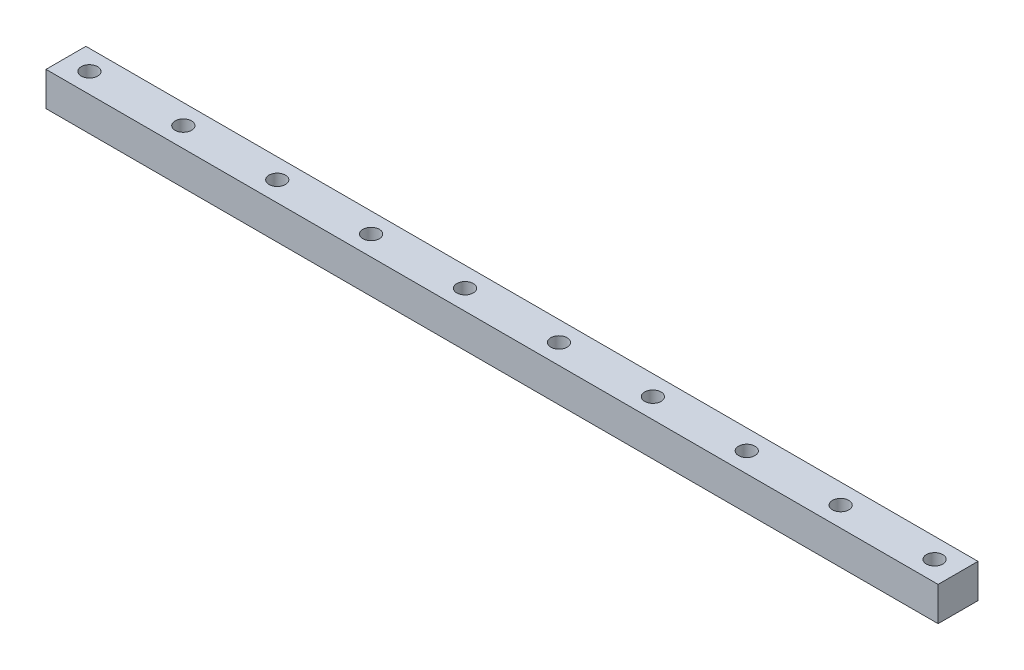
SolidWorks part; units mm, degrees
ref_plane "前视基准面" through (0, 0, 0) normal (0, 0, 1) x (1, 0, 0)
ref_plane "上视基准面" through (0, 0, 0) normal (0, 1, 0) x (1, 0, 0)
ref_plane "右视基准面" through (0, 0, 0) normal (1, 0, 0) x (0, 0, -1)
sketch "草图1" plane through (0, 0, 0) normal (0, 1, 0) x (1, 0, 0)
  line L1 (0, 0) -> (760, 0)
  line L2 (0, 0) -> (0, 34)
  line L3 (0, 34) -> (760, 34)
  line L4 (760, 0) -> (760, 34)
  dimension "D1" = 760
  dimension "D2" = 34
extrude "拉伸1" add sketch "草图1" along normal blind 29
sketch "草图2" plane through (0, 29, 0) normal (0, 1, 0) x (-1, 0, 0)
  line L0 (-760, -17) -> (0, -17) construction
  line L1 (-760, 0) -> (-760, -34) construction
  line L2 (0, -34) -> (0, 0) construction
  line L3 (-20, -34) -> (-20, 0) construction
  line L4 (-760, -34) -> (0, -34) construction
  line L5 (0, 0) -> (-760, 0) construction
  circle A0 centre (-20, -17) radius 7
  dimension "D1" = 20
extrude "切除-拉伸1" cut sketch "草图2" against normal blind 12
sketch "草图3" plane through (0, 17, 0) normal (0, 1, 0) x (-1, 0, 0)
  circle A0 centre (-20, -17) radius 4.5
extrude "切除-拉伸2" cut sketch "草图3" against normal through all
pattern_linear "阵列(线性)1" count 10 spacing 80 along (1, 0, 0) of "切除-拉伸1", "切除-拉伸2"
